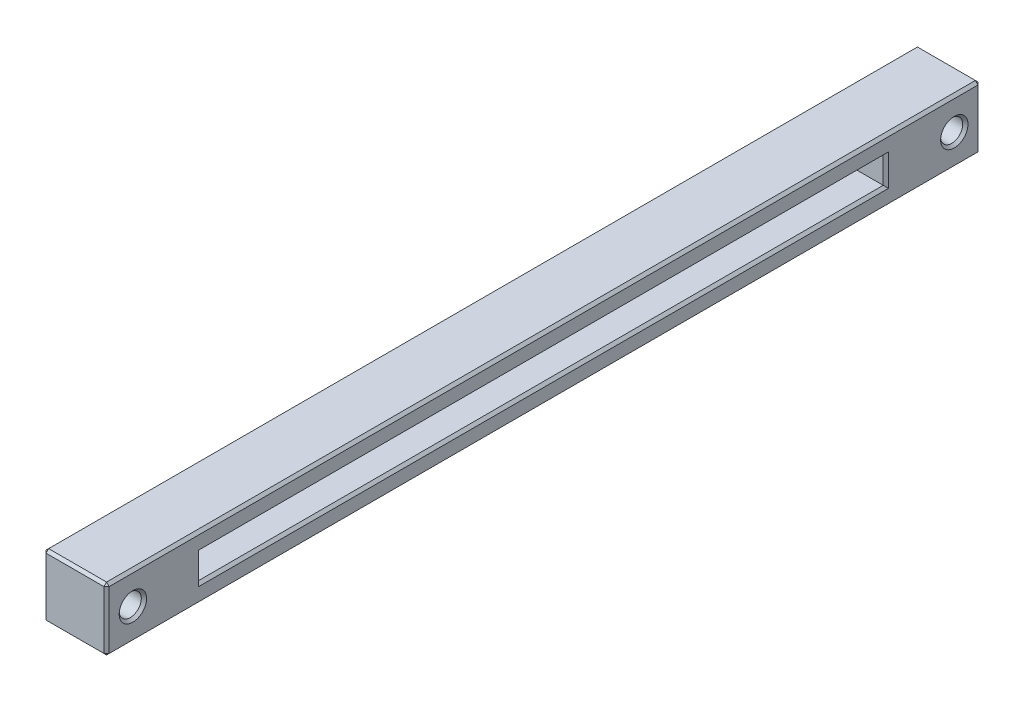
from build123d import *

# Parameters (mm, degrees)
SKETCH_1_W          = 1660
SKETCH_1_H          = 120
EXTRUDE_1_DEPTH     = 120
SKETCH_2_W          = 1300
SKETCH_2_H          = 50
CUT_EXTRUDE_1_DEPTH = 841.773453434
SKETCH_3_R          = 21
CUT_EXTRUDE_2_DEPTH = 841.773453434
CHAMFER_1_SIZE      = 5


with BuildPart() as part:
    # 草图1 → 凸台-拉伸1 (new body)
    with BuildSketch(Plane(origin=(0, 0, 0), x_dir=(0, 0, -1), z_dir=(1, 0, 0))):
        Rectangle(SKETCH_1_W, SKETCH_1_H)
    extrude(amount=EXTRUDE_1_DEPTH)

    # 草图2 → 切除-拉伸1 (cut, through all)
    with BuildSketch(Plane(origin=(120, 0, 0), x_dir=(0, 0, -1), z_dir=(1, 0, 0))):
        Rectangle(SKETCH_2_W, SKETCH_2_H)
    extrude(amount=-CUT_EXTRUDE_1_DEPTH, mode=Mode.SUBTRACT)

    # 草图3 → 切除-拉伸2 (cut, through all)
    with BuildSketch(Plane(origin=(120, 0, 0), x_dir=(0, 0, -1), z_dir=(1, 0, 0))):
        with Locations((-780, 0)):
            Circle(SKETCH_3_R)
        with Locations((780, 0)):
            Circle(SKETCH_3_R)
    extrude(amount=-CUT_EXTRUDE_2_DEPTH, mode=Mode.SUBTRACT)

    # 倒角1
    chamfer_1_edges = [part.edges().sort_by_distance(p)[0] for p in [
        (120, 0, 830),
        (120, -60, 0),
        (0, 0, -650),
        (0, -25, 0),
        (0, 0, 650),
        (0, 25, 0),
        (120, 0, -650),
        (120, 25, 0),
        (120, 0, 650),
        (120, -25, 0),
        (0, 0, 801),
        (120, 0, 801),
        (0, 0, -759),
        (120, 0, -759),
        (120, 0, -830),
        (0, -60, 0),
        (0, 0, 830),
        (0, 60, 0),
        (0, 0, -830),
        (120, 60, 0),
        (60, -60, -830),
        (60, -60, 830),
        (60, 60, 830),
        (60, 60, -830),
    ]]
    chamfer(chamfer_1_edges, length=CHAMFER_1_SIZE)


solid = part.part
